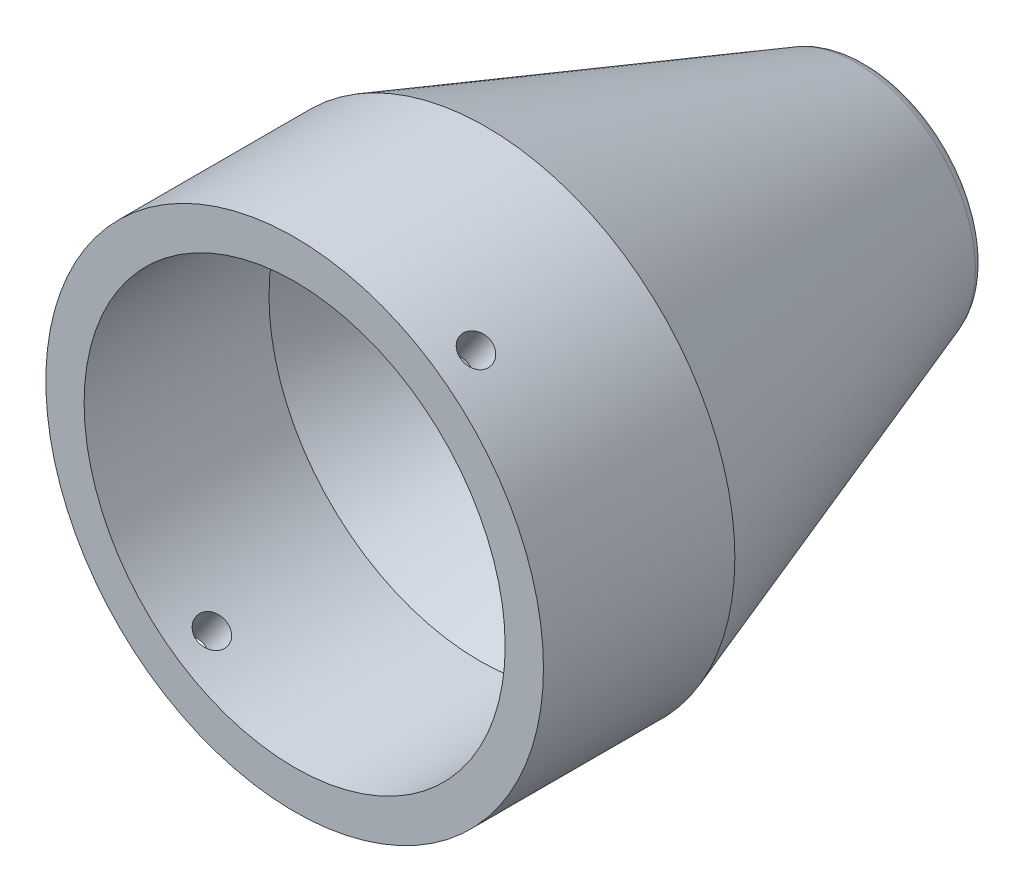
SolidWorks part; units mm, degrees
ref_plane "Front Plane" through (0, 0, 0) normal (0, 0, 1) x (1, 0, 0)
ref_plane "Top Plane" through (0, 0, 0) normal (0, 1, 0) x (1, 0, 0)
ref_plane "Right Plane" through (0, 0, 0) normal (1, 0, 0) x (0, 0, -1)
ref_plane "Plane1" through (0, 234.744, 0) normal (0, 1, 0) x (1, 0, 0)
sketch "Sketch1" plane through (0, 234.744, 0) normal (0, 1, 0) x (1, 0, 0)
  line L0 (551.2306, 1664.9984) -> (521.2306, 1664.9984)
  line L1 (521.2306, 1664.9984) -> (521.2306, 1514.9984)
  line L2 (521.2306, 1514.9984) -> (586.2306, 1514.9984)
  line L3 (586.2306, 1514.9984) -> (586.2306, 1564.9984)
  line L4 (586.2306, 1564.9984) -> (551.2306, 1664.9984)
  line L5 (521.2306, 1664.9984) -> (521.2306, 1514.9984) construction
  dimension "D1" = 30
  dimension "D2" = 65
  dimension "D3" = 50
  dimension "D4" = 150
revolve "Revolve1" add sketch "Sketch1" angle 360 about L5
hole_wizard "M100 clearance hole1" positions "Sketch3" profile "Sketch2" hole size "M100" standard "ANSI Metric"
sketch "Sketch3" plane through (0, 0, -1514.9984) normal (0, 0, 1) x (1, 0, 0)
  point P0 (521.2306, 234.744)
sketch "Sketch2" plane through (521.2306, 234.744, -1514.9984) normal (1, 0, 0) x (0, -1, 0)
  line L0 (0, 0) -> (0, 205.4434)
  line L1 (0, 205.4434) -> (55, 48.3005)
  line L2 (55, 48.3005) -> (55, 0)
  line L5 (55, 0) -> (0, 0)
  line L10 (0, 205.4434) -> (-55, 48.3005) construction
  line L11 (0, -6.35) -> (0, 107.95) construction
  dimension "孔直径" = 110
  dimension "孔深度" = 48.3005
  dimension "导头角度" = 38.58
hole_wizard "Ø8.0 (8) diameter hole1" positions "3D sketch1" profile "Sketch4" hole size "Ø8.0" standard "ANSI Metric"
sketch3d "3D sketch1"
  point P0 (558.6307, 287.9063, -1524.9984)
sketch "Sketch4" plane through (558.6307, 287.9063, -1524.9984) normal (0, 0, 1) x (-0.8179, 0.5754, 0)
  line L0 (0, 0) -> (0, 140.1456)
  line L1 (0, 140.1456) -> (4, 140.1456)
  line L2 (4, 140.1456) -> (4, 0)
  line L5 (4, 0) -> (0, 0)
  line L10 (0, 140.1456) -> (-4, 140.1456) construction
  line L11 (0, -6.35) -> (0, 107.95) construction
  dimension "孔直径" = 8
  dimension "孔深度" = 140.1456
  dimension "导头角度" = 180
fillet "Fillet1" radius 5 1 edges at (551.2306, 234.744, -1664.9984)
